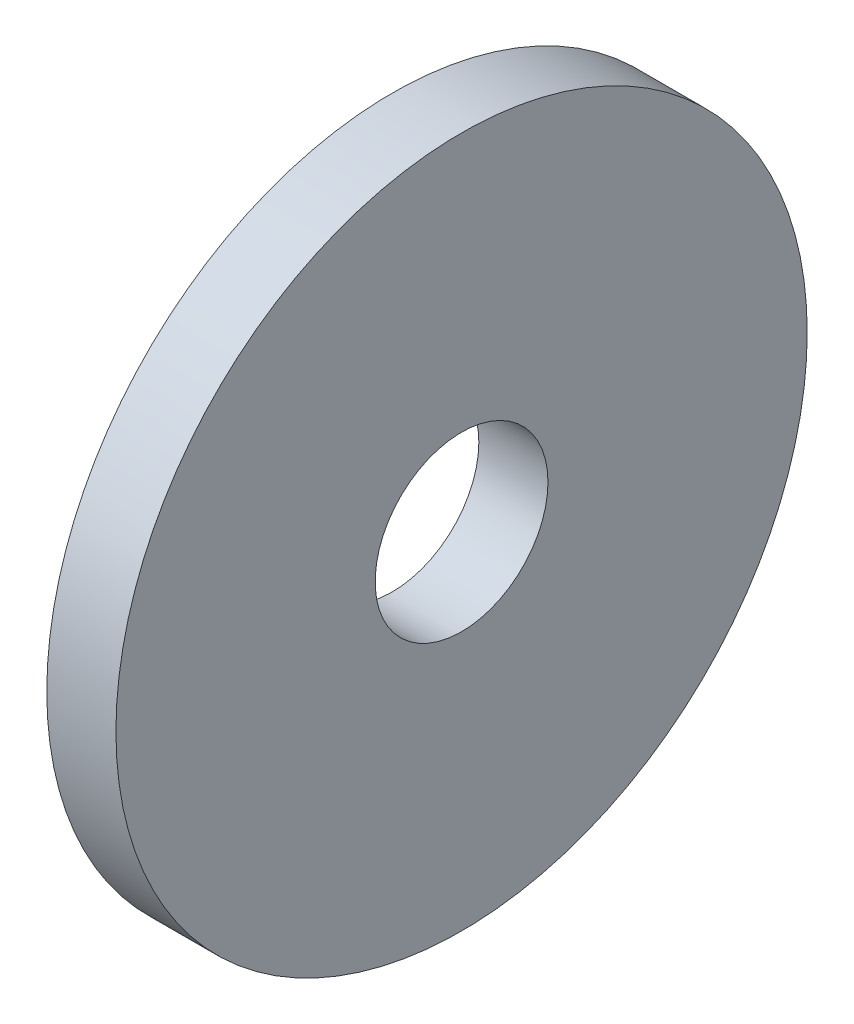
from build123d import *

# Parameters (mm, degrees)
SKETCH1_R           = 20
SKETCH1_R_2         = 5
BOSS_EXTRUDE1_DEPTH = 2


with BuildPart() as part:
    # Sketch1 → Boss-Extrude1 (new, symmetric)
    with BuildSketch(Plane(origin=(0, 0, 0), x_dir=(0, 0, -1), z_dir=(1, 0, 0))):
        Circle(SKETCH1_R)
        Circle(SKETCH1_R_2, mode=Mode.SUBTRACT)
    extrude(amount=BOSS_EXTRUDE1_DEPTH, both=True)


solid = part.part
